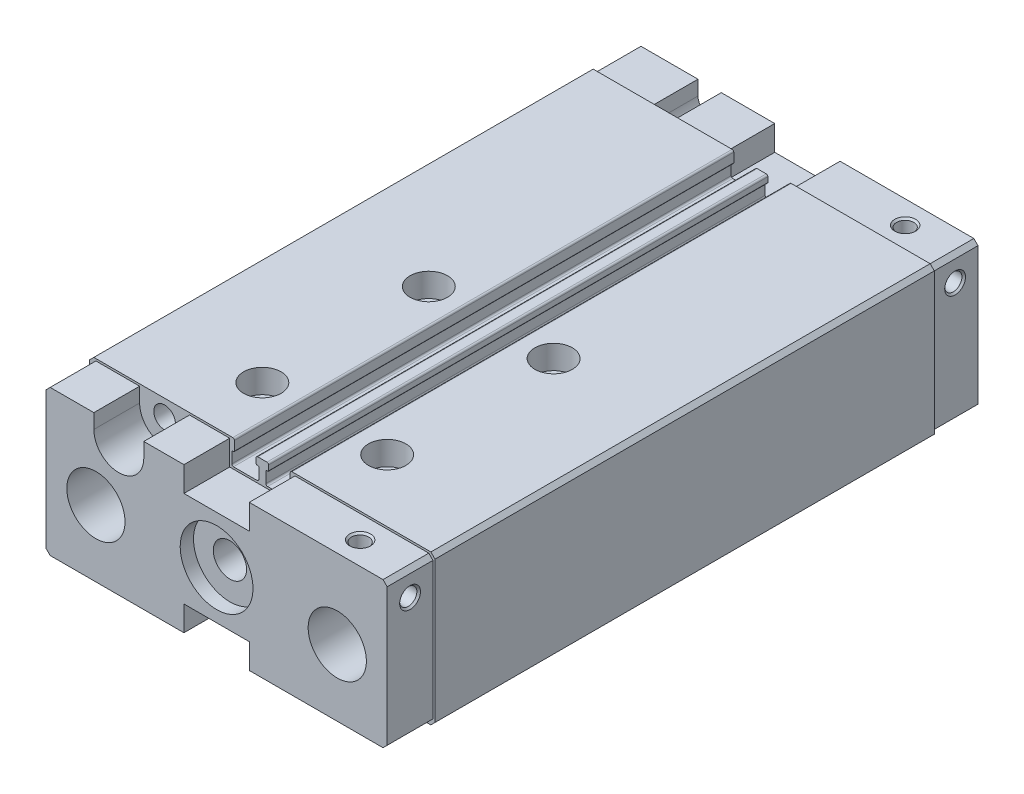
from build123d import *

# Parameters (mm, degrees)
BOSS_EXTRUDE1_DEPTH = 120
BOSS_EXTRUDE2_DEPTH = 11
BOSS_EXTRUDE3_DEPTH = 11
CUT_EXTRUDE1_DEPTH  = 11
CUT_EXTRUDE2_DEPTH  = 11
SKETCH14_W          = 1.6
SKETCH14_H          = 3.5
SKETCH15_W          = 1.6
SKETCH15_H          = 3.5
SKETCH22_W          = 7
SKETCH22_H          = 142
SKETCH28_W          = 142
SKETCH28_H          = 2.6
SKETCH29_W          = 30
SKETCH29_H          = 4
SKETCH30_W          = 7
SKETCH30_H          = 142


with BuildPart() as part:
    # Sketch1 → Boss-Extrude1 (new body)
    with BuildSketch(Plane.XY.offset(-11)):
        with BuildLine():
            Line((-41.5, -17), (-40.5, -18))
            Line((-40.5, -18), (-7.2, -18))
            Line((-7.2, -18), (-6.7, -17.5))
            Line((-6.7, -17.5), (-6.7, -15.4))
            ThreePointArc((-6.7, -15.4), (-6.758578644, -15.258578644), (-6.9, -15.2))
            Line((-6.9, -15.2), (-7.15, -15.2))
            ThreePointArc((-7.15, -15.2), (-7.291421356, -15.141421356), (-7.35, -15))
            Line((-7.35, -15), (-7.35, -12.4))
            ThreePointArc((-7.35, -12.4), (-7.232842712, -12.117157288), (-6.95, -12))
            Line((-6.95, -12), (-1.25, -12))
            ThreePointArc((-1.25, -12), (-0.967157288, -12.117157288), (-0.85, -12.4))
            Line((-0.85, -12.4), (-0.85, -15))
            ThreePointArc((-0.85, -15), (-0.908578644, -15.141421356), (-1.05, -15.2))
            Line((-1.05, -15.2), (-1.3, -15.2))
            ThreePointArc((-1.3, -15.2), (-1.441421356, -15.258578644), (-1.5, -15.4))
            Line((-1.5, -15.4), (-1.5, -16.6))
            ThreePointArc((-1.5, -16.6), (-1.382842712, -16.882842712), (-1.1, -17))
            Line((-1.1, -17), (1.1, -17))
            ThreePointArc((1.1, -17), (1.382842712, -16.882842712), (1.5, -16.6))
            Line((1.5, -16.6), (1.5, -15.4))
            ThreePointArc((1.5, -15.4), (1.441421356, -15.258578644), (1.3, -15.2))
            Line((1.3, -15.2), (1.05, -15.2))
            ThreePointArc((1.05, -15.2), (0.908578644, -15.141421356), (0.85, -15))
            Line((0.85, -15), (0.85, -12.4))
            ThreePointArc((0.85, -12.4), (0.967157288, -12.117157288), (1.25, -12))
            Line((1.25, -12), (6.95, -12))
            ThreePointArc((6.95, -12), (7.232842712, -12.117157288), (7.35, -12.4))
            Line((7.35, -12.4), (7.35, -15))
            ThreePointArc((7.35, -15), (7.291421356, -15.141421356), (7.15, -15.2))
            Line((7.15, -15.2), (6.9, -15.2))
            ThreePointArc((6.9, -15.2), (6.758578644, -15.258578644), (6.7, -15.4))
            Line((6.7, -15.4), (6.7, -17.5))
            Line((6.7, -17.5), (7.2, -18))
            Line((7.2, -18), (40.5, -18))
            Line((40.5, -18), (41.5, -17))
            Line((41.5, -17), (41.5, 17))
            Line((41.5, 17), (40.5, 18))
            Line((40.5, 18), (7.1, 18))
            ThreePointArc((7.1, 18), (6.817157288, 17.882842712), (6.7, 17.6))
            Line((6.7, 17.6), (6.7, 15.4))
            ThreePointArc((6.7, 15.4), (6.758578644, 15.258578644), (6.9, 15.2))
            Line((6.9, 15.2), (7.15, 15.2))
            ThreePointArc((7.15, 15.2), (7.291421356, 15.141421356), (7.35, 15))
            Line((7.35, 15), (7.35, 12.4))
            ThreePointArc((7.35, 12.4), (7.232842712, 12.117157288), (6.95, 12))
            Line((6.95, 12), (1.25, 12))
            ThreePointArc((1.25, 12), (0.967157288, 12.117157288), (0.85, 12.4))
            Line((0.85, 12.4), (0.85, 15))
            ThreePointArc((0.85, 15), (0.908578644, 15.141421356), (1.05, 15.2))
            Line((1.05, 15.2), (1.3, 15.2))
            ThreePointArc((1.3, 15.2), (1.441421356, 15.258578644), (1.5, 15.4))
            Line((1.5, 15.4), (1.5, 16.6))
            ThreePointArc((1.5, 16.6), (1.382842712, 16.882842712), (1.1, 17))
            Line((1.1, 17), (-1.1, 17))
            ThreePointArc((-1.1, 17), (-1.382842712, 16.882842712), (-1.5, 16.6))
            Line((-1.5, 16.6), (-1.5, 15.4))
            ThreePointArc((-1.5, 15.4), (-1.441421356, 15.258578644), (-1.3, 15.2))
            Line((-1.3, 15.2), (-1.05, 15.2))
            ThreePointArc((-1.05, 15.2), (-0.908578644, 15.141421356), (-0.85, 15))
            Line((-0.85, 15), (-0.85, 12.4))
            ThreePointArc((-0.85, 12.4), (-0.967157288, 12.117157288), (-1.25, 12))
            Line((-1.25, 12), (-6.95, 12))
            ThreePointArc((-6.95, 12), (-7.232842712, 12.117157288), (-7.35, 12.4))
            Line((-7.35, 12.4), (-7.35, 15))
            ThreePointArc((-7.35, 15), (-7.291421356, 15.141421356), (-7.15, 15.2))
            Line((-7.15, 15.2), (-6.9, 15.2))
            ThreePointArc((-6.9, 15.2), (-6.758578644, 15.258578644), (-6.7, 15.4))
            Line((-6.7, 15.4), (-6.7, 17.6))
            ThreePointArc((-6.7, 17.6), (-6.817157288, 17.882842712), (-7.1, 18))
            Line((-7.1, 18), (-40.5, 18))
            Line((-40.5, 18), (-41.5, 17))
            Line((-41.5, 17), (-41.5, -17))
        make_face()
    extrude(amount=-BOSS_EXTRUDE1_DEPTH)

    # Sketch2 → Boss-Extrude2 (add)
    with BuildSketch(Plane.XY.offset(-142)):
        Polygon((-41, -16.5), (-40, -17.5), (-7.85, -17.5), (-7.85, -11.5), (7.85, -11.5), (7.85, -17.5), (40, -17.5), (41, -16.5), (41, 16.5), (40, 17.5), (7.85, 17.5), (7.85, 11.5), (-7.85, 11.5), (-7.85, 17.5), (-40, 17.5), (-41, 16.5), align=None)
    extrude(amount=BOSS_EXTRUDE2_DEPTH)

    # Sketch3 → Boss-Extrude3 (add)
    with BuildSketch(Plane.XY):
        Polygon((-41, -16.5), (-40, -17.5), (-7.85, -17.5), (-7.85, -11.5), (7.85, -11.5), (7.85, -17.5), (40, -17.5), (41, -16.5), (41, 16.5), (40, 17.5), (7.85, 17.5), (7.85, 11.5), (-7.85, 11.5), (-7.85, 17.5), (-40, 17.5), (-41, 16.5), align=None)
    extrude(amount=-BOSS_EXTRUDE3_DEPTH)

    # Sketch4 → Cut-Revolve1 (revolve, cut)
    with BuildSketch(Plane.XY.offset(-26), mode=Mode.PRIVATE) as cut_revolve1_sk:
        Polygon((15, 18), (19.5, 18), (19.5, 12.3), (17.65, 12.3), (17.65, -6), (16, -6), (16, -15.9), (19.5, -15.9), (19.5, -18), (15, -18), align=None)
    revolve(cut_revolve1_sk.sketch.rotate(Axis((15, -18, -26), (0, 1, 0)), 270), axis=Axis((15, -18, -26), (0, 1, 0)), mode=Mode.SUBTRACT)

    # Sketch5 → Cut-Revolve2 (revolve, cut)
    with BuildSketch(Plane.XY.offset(-26), mode=Mode.PRIVATE) as cut_revolve2_sk:
        Polygon((15, -6), (17.4585, -6), (17.4585, -15.3585), (18, -15.9), (15, -15.9), align=None)
    revolve(cut_revolve2_sk.sketch.rotate(Axis((15, -15.9, -26), (0, 1, 0)), 270), axis=Axis((15, -15.9, -26), (0, 1, 0)), mode=Mode.SUBTRACT)

    # Sketch6 → Cut-Revolve3 (revolve, cut)
    with BuildSketch(Plane.XY.offset(-26), mode=Mode.PRIVATE) as cut_revolve3_sk:
        Polygon((-15, 18), (-10.5, 18), (-10.5, 12.3), (-12.35, 12.3), (-12.35, -6), (-14, -6), (-14, -15.9), (-10.5, -15.9), (-10.5, -18), (-15, -18), align=None)
    revolve(cut_revolve3_sk.sketch.rotate(Axis((-15, -18, -26), (0, 1, 0)), 270), axis=Axis((-15, -18, -26), (0, 1, 0)), mode=Mode.SUBTRACT)

    # Sketch7 → Cut-Revolve4 (revolve, cut)
    with BuildSketch(Plane.XY.offset(-26), mode=Mode.PRIVATE) as cut_revolve4_sk:
        Polygon((-15, -6), (-12.5415, -6), (-12.5415, -15.3585), (-12, -15.9), (-15, -15.9), align=None)
    revolve(cut_revolve4_sk.sketch.rotate(Axis((-15, -15.9, -26), (0, 1, 0)), 270), axis=Axis((-15, -15.9, -26), (0, 1, 0)), mode=Mode.SUBTRACT)

    # Sketch8 → Cut-Revolve5 (revolve, cut)
    with BuildSketch(Plane.XY.offset(-66), mode=Mode.PRIVATE) as cut_revolve5_sk:
        Polygon((15, 18), (19.5, 18), (19.5, 12.3), (17.65, 12.3), (17.65, -6), (16, -6), (16, -18), (15, -18), align=None)
    revolve(cut_revolve5_sk.sketch.rotate(Axis((15, -18, -66), (0, 1, 0)), 270), axis=Axis((15, -18, -66), (0, 1, 0)), mode=Mode.SUBTRACT)

    # Sketch9 → Cut-Revolve6 (revolve, cut)
    with BuildSketch(Plane.XY.offset(-66), mode=Mode.PRIVATE) as cut_revolve6_sk:
        Polygon((15, -6), (17.4585, -6), (17.4585, -17.4585), (18, -18), (15, -18), align=None)
    revolve(cut_revolve6_sk.sketch.rotate(Axis((15, -18, -66), (0, 1, 0)), 270), axis=Axis((15, -18, -66), (0, 1, 0)), mode=Mode.SUBTRACT)

    # Sketch10 → Cut-Revolve7 (revolve, cut)
    with BuildSketch(Plane.XY.offset(-66), mode=Mode.PRIVATE) as cut_revolve7_sk:
        Polygon((-15, 18), (-10.5, 18), (-10.5, 12.3), (-12.35, 12.3), (-12.35, -6), (-14, -6), (-14, -18), (-15, -18), align=None)
    revolve(cut_revolve7_sk.sketch.rotate(Axis((-15, -18, -66), (0, 1, 0)), 270), axis=Axis((-15, -18, -66), (0, 1, 0)), mode=Mode.SUBTRACT)

    # Sketch11 → Cut-Revolve8 (revolve, cut)
    with BuildSketch(Plane.XY.offset(-66), mode=Mode.PRIVATE) as cut_revolve8_sk:
        Polygon((-15, -6), (-12.5415, -6), (-12.5415, -17.4585), (-12, -18), (-15, -18), align=None)
    revolve(cut_revolve8_sk.sketch.rotate(Axis((-15, -18, -66), (0, 1, 0)), 270), axis=Axis((-15, -18, -66), (0, 1, 0)), mode=Mode.SUBTRACT)

    # Sketch12 → Cut-Extrude1 (cut)
    with BuildSketch(Plane.XY):
        with BuildLine():
            Line((-29.5, 18), (-29.5, 14))
            ThreePointArc((-29.5, 14), (-23.5, 8), (-17.5, 14))
            Line((-17.5, 14), (-17.5, 18))
            Line((-17.5, 18), (-29.5, 18))
        make_face()
    extrude(amount=-CUT_EXTRUDE1_DEPTH, mode=Mode.SUBTRACT)

    # Sketch13 → Cut-Extrude2 (cut)
    with BuildSketch(Plane.XY.offset(-142)):
        with BuildLine():
            Line((-26.3, 18), (-26.3, 14))
            ThreePointArc((-26.3, 14), (-23.5, 11.2), (-20.7, 14))
            Line((-20.7, 14), (-20.7, 18))
            Line((-20.7, 18), (-26.3, 18))
        make_face()
    extrude(amount=CUT_EXTRUDE2_DEPTH, mode=Mode.SUBTRACT)

    # Sketch14 → Cut-Revolve9 (revolve, cut)
    with BuildSketch(Plane.XY.offset(-26), mode=Mode.PRIVATE) as cut_revolve9_sk:
        with Locations((-40.7, 1.75)):
            Rectangle(SKETCH14_W, SKETCH14_H)
    revolve(cut_revolve9_sk.sketch.rotate(Axis((-39.9, 0, -26), (-1, 0, 0)), 270), axis=Axis((-39.9, 0, -26), (-1, 0, 0)), mode=Mode.SUBTRACT)

    # Sketch15 → Cut-Revolve10 (revolve, cut)
    with BuildSketch(Plane.XY.offset(-66), mode=Mode.PRIVATE) as cut_revolve10_sk:
        with Locations((-40.7, 1.75)):
            Rectangle(SKETCH15_W, SKETCH15_H)
    revolve(cut_revolve10_sk.sketch.rotate(Axis((-39.9, 0, -66), (-1, 0, 0)), 270), axis=Axis((-39.9, 0, -66), (-1, 0, 0)), mode=Mode.SUBTRACT)

    # Sketch16 → Cut-Revolve11 (revolve, cut)
    with BuildSketch(Plane.XY.offset(-26), mode=Mode.PRIVATE) as cut_revolve11_sk:
        Polygon((-41.5, -13.5), (-41.5, -11), (-41.067, -11.433), (-29.360049673, -11.433), (-28.166666667, -13.5), align=None)
    revolve(cut_revolve11_sk.sketch.rotate(Axis((-28.166666667, -13.5, -26), (-1, 0, 0)), 270), axis=Axis((-28.166666667, -13.5, -26), (-1, 0, 0)), mode=Mode.SUBTRACT)

    # Sketch17 → Cut-Revolve12 (revolve, cut)
    with BuildSketch(Plane.XY.offset(-26), mode=Mode.PRIVATE) as cut_revolve12_sk:
        Polygon((-41.5, 13.5), (-41.5, 16), (-41.067, 15.567), (-29.360049673, 15.567), (-28.166666667, 13.5), align=None)
    revolve(cut_revolve12_sk.sketch.rotate(Axis((-28.166666667, 13.5, -26), (-1, 0, 0)), 270), axis=Axis((-28.166666667, 13.5, -26), (-1, 0, 0)), mode=Mode.SUBTRACT)

    # Sketch18 → Cut-Revolve13 (revolve, cut)
    with BuildSketch(Plane.XY.offset(-66), mode=Mode.PRIVATE) as cut_revolve13_sk:
        Polygon((-41.5, -13.5), (-41.5, -11), (-41.067, -11.433), (-29.360049673, -11.433), (-28.166666667, -13.5), align=None)
    revolve(cut_revolve13_sk.sketch.rotate(Axis((-28.166666667, -13.5, -66), (-1, 0, 0)), 270), axis=Axis((-28.166666667, -13.5, -66), (-1, 0, 0)), mode=Mode.SUBTRACT)

    # Sketch19 → Cut-Revolve14 (revolve, cut)
    with BuildSketch(Plane.XY.offset(-66), mode=Mode.PRIVATE) as cut_revolve14_sk:
        Polygon((-41.5, 13.5), (-41.5, 16), (-41.067, 15.567), (-29.360049673, 15.567), (-28.166666667, 13.5), align=None)
    revolve(cut_revolve14_sk.sketch.rotate(Axis((-28.166666667, 13.5, -66), (-1, 0, 0)), 270), axis=Axis((-28.166666667, 13.5, -66), (-1, 0, 0)), mode=Mode.SUBTRACT)

    # Sketch20 → Cut-Revolve15 (revolve, cut)
    with BuildSketch(Plane(origin=(29, 0, 0), x_dir=(0, 0, -1), z_dir=(1, 0, 0))):
        Polygon((5.5, 12.5), (3.433, 12.5), (3.433, 17.067), (3, 17.5), (5.5, 17.5), align=None)
    revolve(axis=Axis((29, 17.5, -5.5), (0, -1, 0)), mode=Mode.SUBTRACT)

    # Sketch21 → Cut-Revolve16 (revolve, cut)
    with BuildSketch(Plane(origin=(29, 0, 0), x_dir=(0, 0, -1), z_dir=(1, 0, 0))):
        Polygon((136.5, 12.5), (134.433, 12.5), (134.433, 17.067), (134, 17.5), (136.5, 17.5), align=None)
    revolve(axis=Axis((29, 17.5, -136.5), (0, -1, 0)), mode=Mode.SUBTRACT)

    # Sketch22 → Cut-Revolve17 (revolve, cut)
    with BuildSketch(Plane(origin=(0, -1.5, 0), x_dir=(1, 0, 0), z_dir=(0, 1, 0)), mode=Mode.PRIVATE) as cut_revolve17_sk:
        with Locations((32.5, 71)):
            Rectangle(SKETCH22_W, SKETCH22_H)
    revolve(cut_revolve17_sk.sketch.rotate(Axis((29, -1.5, 0), (0, 0, -1)), 180), axis=Axis((29, -1.5, 0), (0, 0, -1)), mode=Mode.SUBTRACT)

    # Sketch23 → Cut-Revolve18 (revolve, cut)
    with BuildSketch(Plane(origin=(0, 11.5, 0), x_dir=(1, 0, 0), z_dir=(0, 1, 0)), mode=Mode.PRIVATE) as cut_revolve18_sk:
        Polygon((36, 5.5), (36, 7.567), (40.567, 7.567), (41, 8), (41, 5.5), align=None)
    revolve(cut_revolve18_sk.sketch.rotate(Axis((41, 11.5, -5.5), (-1, 0, 0)), 180), axis=Axis((41, 11.5, -5.5), (-1, 0, 0)), mode=Mode.SUBTRACT)

    # Sketch24 → Cut-Revolve19 (revolve, cut)
    with BuildSketch(Plane(origin=(0, 11.5, 0), x_dir=(1, 0, 0), z_dir=(0, 1, 0)), mode=Mode.PRIVATE) as cut_revolve19_sk:
        Polygon((36, 136.5), (36, 138.567), (40.567, 138.567), (41, 139), (41, 136.5), align=None)
    revolve(cut_revolve19_sk.sketch.rotate(Axis((41, 11.5, -136.5), (-1, 0, 0)), 180), axis=Axis((41, 11.5, -136.5), (-1, 0, 0)), mode=Mode.SUBTRACT)

    # Sketch25 → Cut-Revolve20 (revolve, cut)
    with BuildSketch(Plane(origin=(0, -13.5, 0), x_dir=(1, 0, 0), z_dir=(0, 1, 0)), mode=Mode.PRIVATE) as cut_revolve20_sk:
        Polygon((35, 142), (37.5, 142), (37.067, 141.567), (37.067, 131), (35, 131), align=None)
    revolve(cut_revolve20_sk.sketch.rotate(Axis((35, -13.5, -131), (0, 0, -1)), 180), axis=Axis((35, -13.5, -131), (0, 0, -1)), mode=Mode.SUBTRACT)

    # Sketch26 → Cut-Revolve21 (revolve, cut)
    with BuildSketch(Plane(origin=(0, 13.5, 0), x_dir=(1, 0, 0), z_dir=(0, 1, 0)), mode=Mode.PRIVATE) as cut_revolve21_sk:
        Polygon((-35, 142), (-32.5, 142), (-32.933, 141.567), (-32.933, 131), (-35, 131), align=None)
    revolve(cut_revolve21_sk.sketch.rotate(Axis((-35, 13.5, -131), (0, 0, -1)), 180), axis=Axis((-35, 13.5, -131), (0, 0, -1)), mode=Mode.SUBTRACT)

    # Sketch27 → Cut-Revolve22 (revolve, cut)
    with BuildSketch(Plane(origin=(0, 0, 0), x_dir=(0, 0, -1), z_dir=(1, 0, 0)), mode=Mode.PRIVATE) as cut_revolve22_sk:
        Polygon((0, 0), (0, 8.75), (3.2, 8.75), (3.2, 4), (22, 4), (22, 10), (112, 10), (112, 0), align=None)
    revolve(cut_revolve22_sk.sketch.rotate(Axis((0, 0, -112), (0, 0, 1)), 90), axis=Axis((0, 0, -112), (0, 0, 1)), mode=Mode.SUBTRACT)

    # Sketch28 → Cut-Revolve23 (revolve, cut)
    with BuildSketch(Plane(origin=(-23.5, 0, 0), x_dir=(0, 0, -1), z_dir=(1, 0, 0)), mode=Mode.PRIVATE) as cut_revolve23_sk:
        with Locations((71, 15.3)):
            Rectangle(SKETCH28_W, SKETCH28_H)
    revolve(cut_revolve23_sk.sketch.rotate(Axis((-23.5, 14, -142), (0, 0, 1)), 270), axis=Axis((-23.5, 14, -142), (0, 0, 1)), mode=Mode.SUBTRACT)

    # Sketch29 → Cut-Revolve24 (revolve, cut)
    with BuildSketch(Plane(origin=(0, 0, 0), x_dir=(0, 0, -1), z_dir=(1, 0, 0)), mode=Mode.PRIVATE) as cut_revolve24_sk:
        with Locations((127, 2)):
            Rectangle(SKETCH29_W, SKETCH29_H)
    revolve(cut_revolve24_sk.sketch.rotate(Axis((0, 0, -142), (0, 0, 1)), 90), axis=Axis((0, 0, -142), (0, 0, 1)), mode=Mode.SUBTRACT)

    # Sketch30 → Cut-Revolve25 (revolve, cut)
    with BuildSketch(Plane(origin=(0, -1.5, 0), x_dir=(1, 0, 0), z_dir=(0, 1, 0)), mode=Mode.PRIVATE) as cut_revolve25_sk:
        with Locations((-25.5, 71)):
            Rectangle(SKETCH30_W, SKETCH30_H)
    revolve(cut_revolve25_sk.sketch.rotate(Axis((-29, -1.5, 0), (0, 0, -1)), 180), axis=Axis((-29, -1.5, 0), (0, 0, -1)), mode=Mode.SUBTRACT)


solid = part.part
